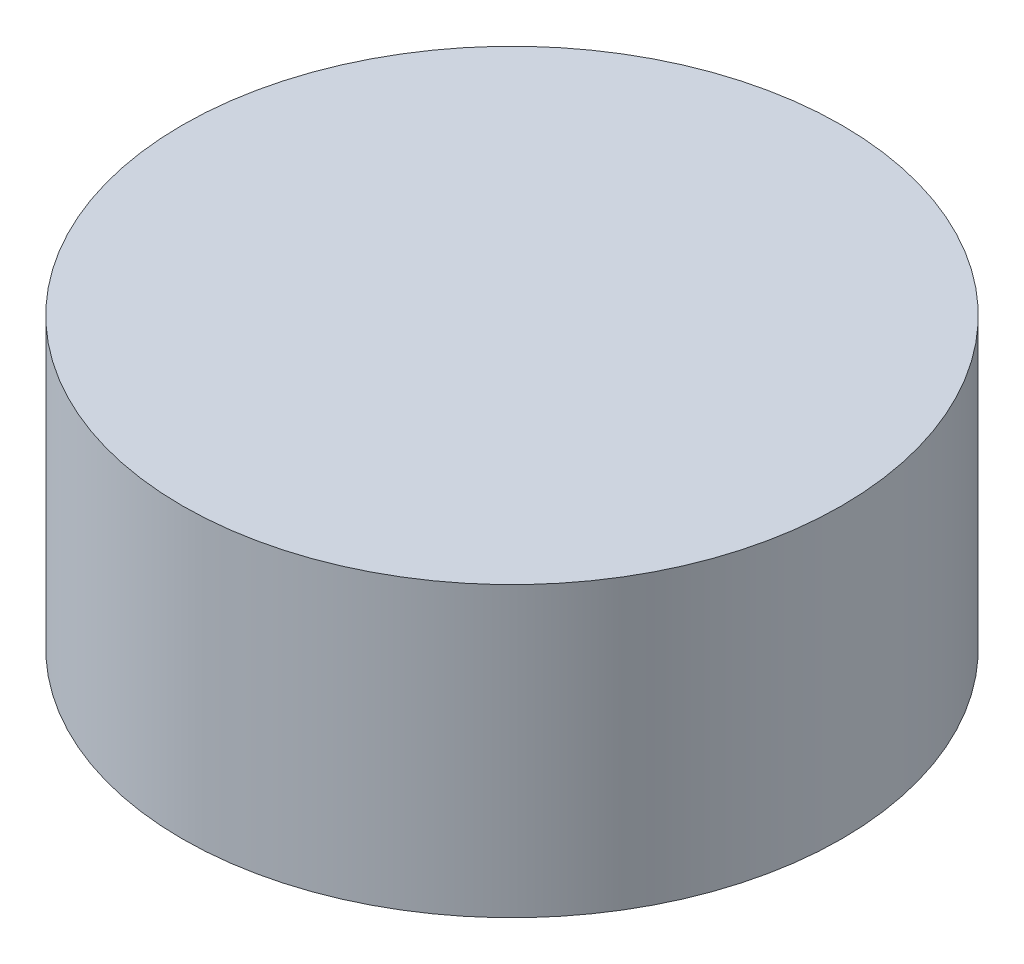
from build123d import *

# Parameters (mm, degrees)
SKETCH1_R           = 16
BOSS_EXTRUDE1_DEPTH = 14


with BuildPart() as part:
    # Sketch1 → Boss-Extrude1 (new body)
    with BuildSketch(Plane(origin=(0, 0, 0), x_dir=(1, 0, 0), z_dir=(0, 1, 0))):
        with Locations(Location((0, 0, 0), (0, 0, 270))):
            Circle(SKETCH1_R)
    extrude(amount=BOSS_EXTRUDE1_DEPTH)


solid = part.part
